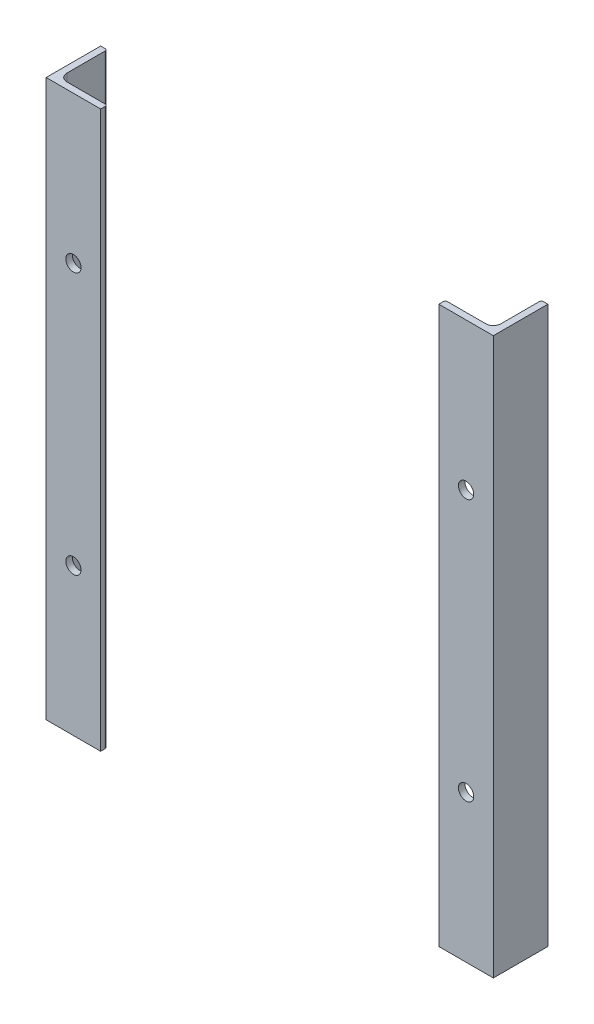
SolidWorks part; units mm, degrees
material "Q235"
ref_plane "Front Plane" through (0, 0, 0) normal (0, 0, 1) x (1, 0, 0)
ref_plane "Top Plane" through (0, 0, 0) normal (0, 1, 0) x (1, 0, 0)
ref_plane "Right Plane" through (0, 0, 0) normal (1, 0, 0) x (0, 0, -1)
sketch "Sketch3" plane through (0, 0, 0) normal (0, 0, 1) x (1, 0, 0)
  line L1 (-102.5, -127.5) -> (102.5, -127.5)
  line L2 (-102.5, -127.5) -> (-102.5, 127.5)
  line L3 (-102.5, 127.5) -> (102.5, 127.5)
  line L4 (102.5, -127.5) -> (102.5, 127.5)
  line L5 (-102.5, -127.5) -> (102.5, 127.5) construction
  line L6 (-102.5, 127.5) -> (102.5, -127.5) construction
  point P0 (0, 0)
  dimension "D1" = 255
  dimension "D2" = 205
other "Equal Angle 2.5X3(1)"
ref_plane "Plane1" through (-102.5, -127.5, 0) normal (0, 1, 0) x (0, 0, -1)
sketch "Sketch1" plane through (-102.5, -127.5, 0) normal (0, 1, 0) x (0, 0, -1)
  line L0 (25, 0) -> (0, 0)
  line L1 (0, 0) -> (0, -25)
  line L2 (24, -3) -> (6.5, -3)
  line L3 (3, -6.5) -> (3, -24)
  line L4 (25, 0) -> (25, -2)
  line L5 (0, -25) -> (2, -25)
  arc A0 (25, -2) -> (24, -3) centre (24, -2) cw
  arc A1 (2, -25) -> (3, -24) centre (2, -24) ccw
  arc A2 (6.5, -3) -> (3, -6.5) centre (6.5, -6.5) ccw
  point P2 (12.5, 0)
  point P13 (0, -12.5)
  point P15 (0, 0)
  dimension "r1" = 1
  dimension "r" = 3.5
  dimension "b" = 25
  dimension "d" = 3
hole_wizard "M6 Clearance Hole1" positions "Sketch5" profile "Sketch6" hole size "M6" standard "GB"
sketch "Sketch5" plane through (0, 0, 0) normal (0, 0, 1) x (1, 0, 0)
  line L0 (0, 0) -> (0, 22.8494) construction
  line L2 (0, 0) -> (-41.8083, 0) construction
  point P0 (-90, 60)
  point P2 (-90, -60)
  point P9 (90, -60)
  point P10 (90, 60)
  dimension "D1" = 120
  dimension "D2" = 180
sketch "Sketch6" plane through (-90, 60, 0) normal (1, 0, 0) x (0, -1, 0)
  line L0 (0, 0) -> (0, 22.103)
  line L1 (0, 22.103) -> (3.5, 20)
  line L2 (3.5, 20) -> (3.5, 0)
  line L5 (3.5, 0) -> (0, 0)
  line L10 (0, 22.103) -> (-3.5, 20) construction
  line L11 (0, -6.35) -> (0, 107.95) construction
  dimension "孔直径" = 7
  dimension "孔深度" = 20
  dimension "导头角度" = 118
